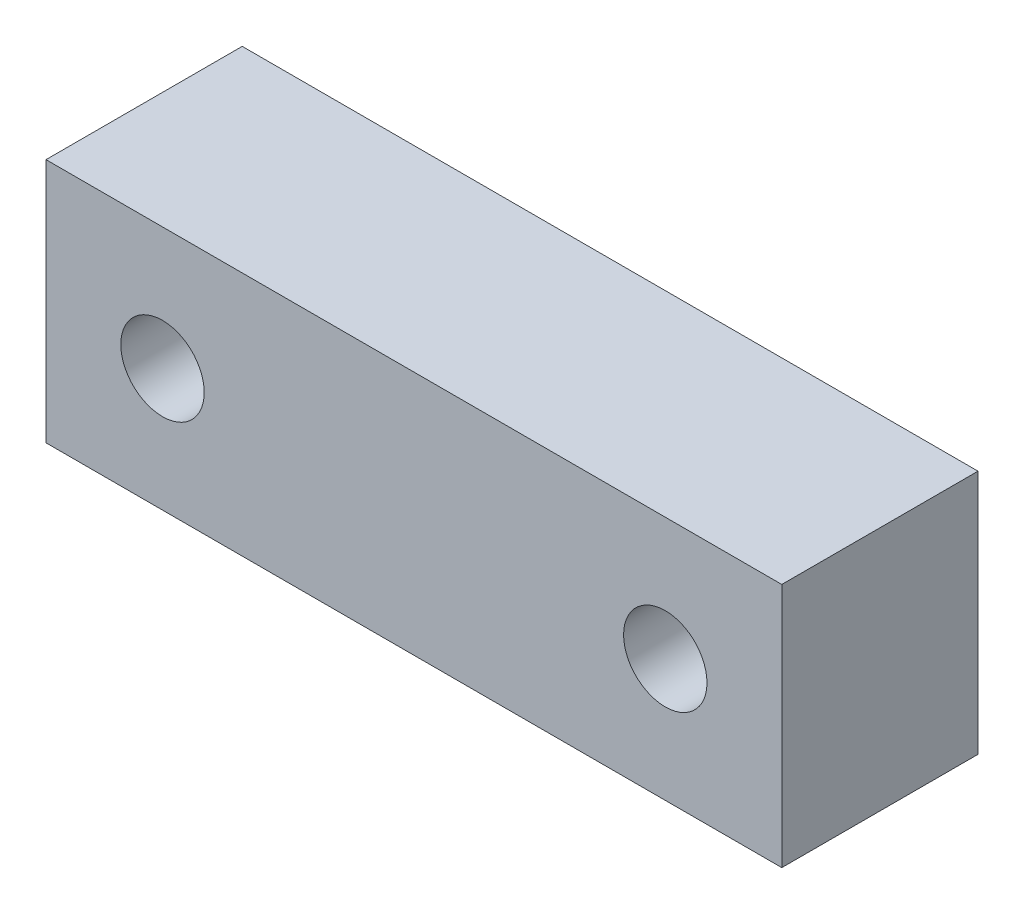
from build123d import *

# Parameters (mm, degrees)
SKETCH_1_W                = 30
SKETCH_1_H                = 10
EXTRUDE_1_DEPTH           = 8
HOLE_WIZARD_1_D           = 3.4
HOLE_WIZARD_1_CBORE_D     = 6
HOLE_WIZARD_1_CBORE_DEPTH = 3.4


with BuildPart() as part:
    # 草图1 → 凸台-拉伸1 (new body)
    with BuildSketch(Plane.XY):
        Rectangle(SKETCH_1_W, SKETCH_1_H)
    extrude(amount=EXTRUDE_1_DEPTH)

    # 打孔尺寸(%根据)内六角圆柱头螺钉的类型1 (through all)
    with Locations(Plane(origin=(0, 0, 0), x_dir=(-1, 0, 0), z_dir=(0, 0, -1))):
        with Locations((-10.25, 0), (10.25, 0)):
            CounterBoreHole(HOLE_WIZARD_1_D / 2, HOLE_WIZARD_1_CBORE_D / 2, HOLE_WIZARD_1_CBORE_DEPTH)


solid = part.part
